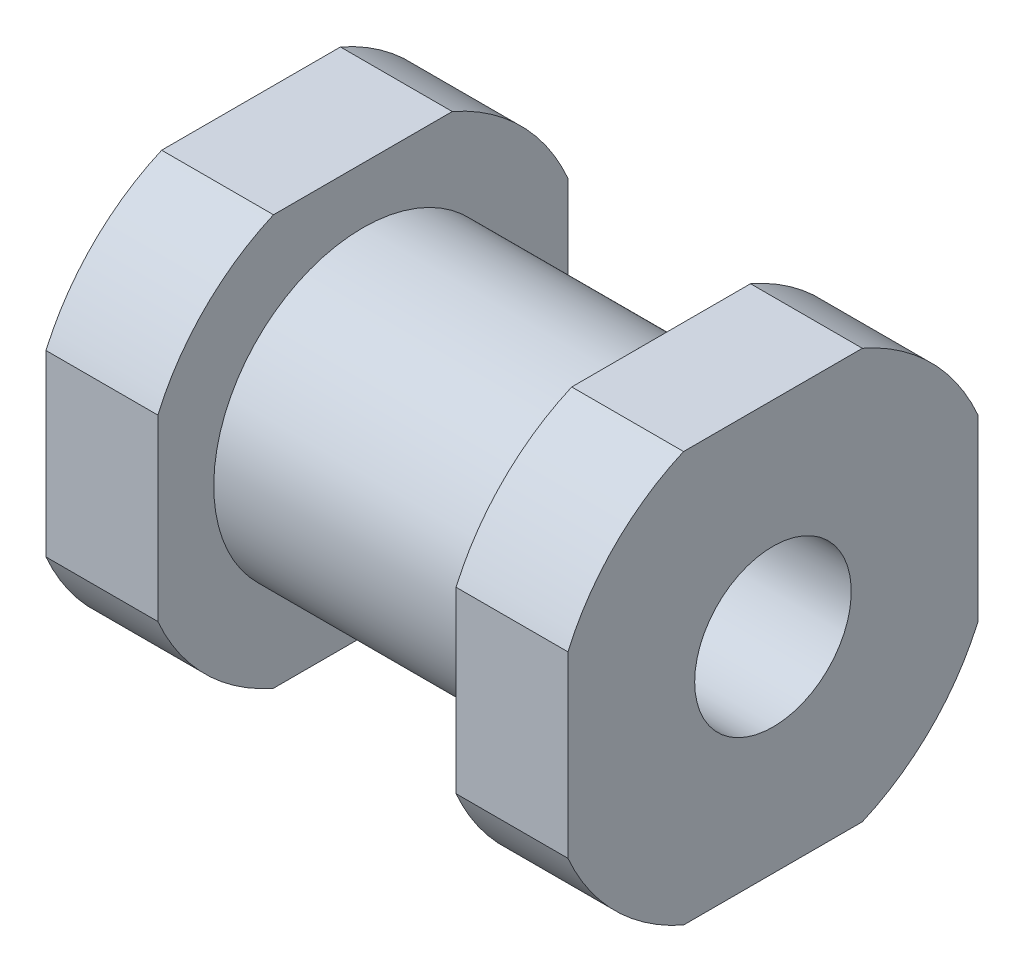
from build123d import *

# Parameters (mm, degrees)
M5_TAPPED_HOLE1_D   = 4.2
SKETCH4_OUTSIDE_W   = 18.4
SKETCH4_OUTSIDE_H   = 18.4
SKETCH4_OUTSIDE_W_2 = 11
SKETCH4_OUTSIDE_H_2 = 11
CUT_EXTRUDE1_DEPTH  = 17.370705544


with BuildPart() as part:
    # Sketch1 → Revolve1 (revolve)
    with BuildSketch(Plane.XY):
        Polygon((0, 6), (0, 0), (14, 0), (14, 6), (11, 6), (11, 4), (3, 4), (3, 6), align=None)
    revolve(axis=Axis((14, 0, 0), (-1, 0, 0)))

    # M5 Tapped Hole1 (through all)
    with Locations(Plane.ZY):
        with Locations((0, 0)):
            Hole(M5_TAPPED_HOLE1_D / 2)

    # Sketch4 outside → Cut-Extrude1 (cut, through all)
    with BuildSketch(Plane.ZY):
        Rectangle(SKETCH4_OUTSIDE_W, SKETCH4_OUTSIDE_H)
        Rectangle(SKETCH4_OUTSIDE_W_2, SKETCH4_OUTSIDE_H_2, mode=Mode.SUBTRACT)
    extrude(amount=-CUT_EXTRUDE1_DEPTH, mode=Mode.SUBTRACT)


solid = part.part
